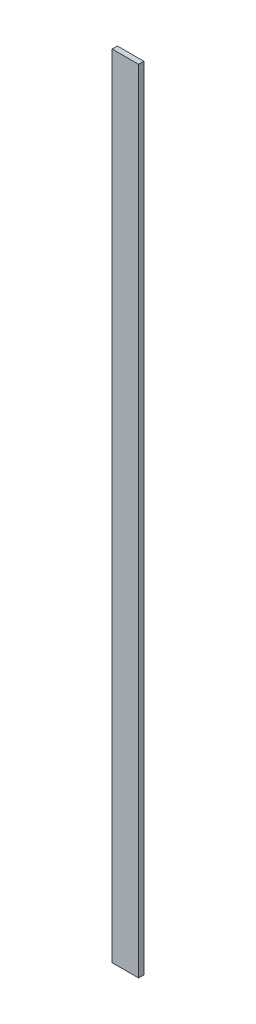
SolidWorks part; units mm, degrees
ref_plane "Front Plane" through (0, 0, 0) normal (0, 0, 1) x (1, 0, 0)
ref_plane "Top Plane" through (0, 0, 0) normal (0, 1, 0) x (1, 0, 0)
ref_plane "Right Plane" through (0, 0, 0) normal (1, 0, 0) x (0, 0, -1)
sketch "Sketch1" plane through (0, 0, 0) normal (0, 0, 1) x (1, 0, 0)
  line L1 (0, 0) -> (10, 0)
  line L2 (0, 0) -> (0, 300)
  line L3 (0, 300) -> (10, 300)
  line L4 (10, 0) -> (10, 300)
  dimension "D1" = 300
  dimension "D2" = 10
extrude "Boss-Extrude1" add sketch "Sketch1" along normal blind 2
